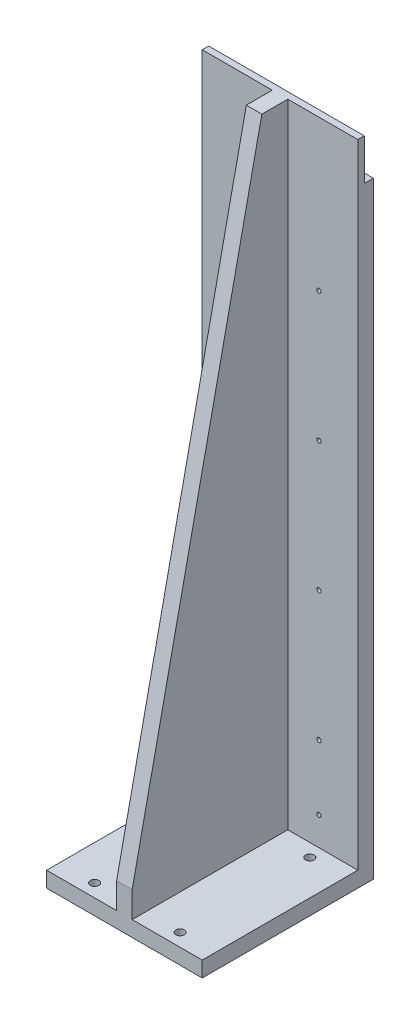
SolidWorks part; units mm, degrees
ref_plane "Front Plane" through (0, 0, 0) normal (0, 0, 1) x (1, 0, 0)
ref_plane "Top Plane" through (0, 0, 0) normal (0, 1, 0) x (1, 0, 0)
ref_plane "Right Plane" through (0, 0, 0) normal (1, 0, 0) x (0, 0, -1)
sketch "Sketch1" plane through (0, 0, 0) normal (0, 0, 1) x (1, 0, 0)
  line L1 (-60, 250) -> (60, 250)
  line L2 (-60, 250) -> (-60, -250)
  line L3 (-60, -250) -> (60, -250)
  line L4 (60, 250) -> (60, -250)
  line L5 (-60, 250) -> (60, -250) construction
  line L6 (-60, -250) -> (60, 250) construction
  point P0 (0, 0)
  dimension "D1" = 120
  dimension "D2" = 500
extrude "Boss-Extrude1" add sketch "Sketch1" along normal blind 12
sketch "Sketch2" plane through (0, 0, 12) normal (0, 0, 1) x (1, 0, 0)
  line L0 (60, -250) -> (60, 250) construction
  line L1 (-60, -250) -> (60, -250)
  line L2 (-60, -250) -> (-60, -238)
  line L3 (-60, -238) -> (60, -238)
  line L4 (60, -250) -> (60, -238)
  dimension "D1" = 12
extrude "Boss-Extrude2" add sketch "Sketch2" along normal blind 120
sketch "Sketch3" plane through (0, 0, 0) normal (1, 0, 0) x (0, 0, -1)
  line L0 (-12, 250) -> (-32, 250)
  line L1 (-12, -238) -> (-12, 250) construction
  line L2 (-32, 250) -> (-132, -218)
  line L3 (-132, -218) -> (-132, -238)
  line L4 (-132, -238) -> (-12, -238) construction
  line L5 (-132, -238) -> (-12, -238)
  line L6 (-12, -238) -> (-12, 250)
  line L8 (-12, 250) -> (0, 250) construction
  dimension "D1" = 20
  dimension "D2" = 20
extrude "Boss-Extrude3" add sketch "Sketch3" along normal mid plane 12
hole_wizard "M6 Clearance Hole1" positions "Sketch5" profile "Sketch4" hole size "M6" standard "GB"
sketch "Sketch5" plane through (0, -238, 0) normal (0, 1, 0) x (1, 0, 0)
  line L1 (33, -122) -> (33, -22) construction
  line L2 (60, -132) -> (60, -12) construction
  line L3 (6, -132) -> (6, -12) construction
  line L4 (60, -12) -> (6, -12) construction
  line L5 (6, -72) -> (33, -72) construction
  point P9 (33, -22)
  point P10 (33, -122)
  dimension "D1" = 10
sketch "Sketch4" plane through (33, -238, 122) normal (1, 0, 0) x (0, 0, 1)
  line L0 (0, 0) -> (0, 16.9828)
  line L1 (0, 16.9828) -> (3.3, 15)
  line L2 (3.3, 15) -> (3.3, 0)
  line L5 (3.3, 0) -> (0, 0)
  line L10 (0, 16.9828) -> (-3.3, 15) construction
  line L11 (0, -6.35) -> (0, 107.95) construction
  dimension "孔直径" = 6.6
  dimension "孔深度" = 15
  dimension "导头角度" = 118
hole_wizard "M6 Clearance Hole2" positions "Sketch7" profile "Sketch6" hole size "M6" standard "GB"
sketch "Sketch7" plane through (0, -238, 0) normal (0, 1, 0) x (1, 0, 0)
  line L1 (-33, -122) -> (-33, -22) construction
  line L2 (-60, -132) -> (-60, -12) construction
  line L3 (-6, -132) -> (-6, -12) construction
  line L4 (-6, -12) -> (-60, -12) construction
  line L5 (-6, -72) -> (-33, -72) construction
  point P9 (-33, -22)
  point P10 (-33, -122)
  dimension "D1" = 10
sketch "Sketch6" plane through (-33, -238, 122) normal (1, 0, 0) x (0, 0, 1)
  line L0 (0, 0) -> (0, 16.9828)
  line L1 (0, 16.9828) -> (3.3, 15)
  line L2 (3.3, 15) -> (3.3, 0)
  line L5 (3.3, 0) -> (0, 0)
  line L10 (0, 16.9828) -> (-3.3, 15) construction
  line L11 (0, -6.35) -> (0, 107.95) construction
  dimension "孔直径" = 6.6
  dimension "孔深度" = 15
  dimension "导头角度" = 118
hole_wizard "M4 Tapped Hole1" positions "Sketch9" profile "Sketch8" tap size "M4" standard "GB" end condition through all
sketch "Sketch9" plane through (0, 0, 0) normal (0, 0, -1) x (-1, 0, 0)
  point P1 (-30, 34)
  point P5 (-30, 134)
  point P9 (-30, -66)
  point P13 (-30, -166)
  point P17 (-30, -216)
  point P21 (30, -216)
  point P25 (30, -166)
  point P29 (30, -66)
  point P33 (30, 34)
  point P37 (30, 134)
  dimension "D1" = 30
  dimension "D2" = 30
  dimension "D3" = 50
  dimension "D4" = 100
  dimension "D5" = 66
  dimension "D6" = 34
  dimension "D7" = 100
sketch "Sketch8" plane through (30, 34, 0) normal (1, 0, 0) x (0, 1, 0)
  line L0 (0, 0) -> (0, 132)
  line L1 (0, 132) -> (1.65, 132)
  line L2 (1.65, 132) -> (1.65, 0)
  line L5 (1.65, 0) -> (0, 0)
  line L11 (0, -6.35) -> (0, 107.95) construction
  dimension "通孔螺纹孔钻头直径" = 3.3
  dimension "通孔螺纹孔钻头深度" = 132
cosmetic thread "Cosmetic Thread3" parameters "D2"=4
cosmetic thread "Cosmetic Thread4" parameters "D2"=4
cosmetic thread "Cosmetic Thread5" parameters "D2"=4
cosmetic thread "Cosmetic Thread6" parameters "D2"=4
cosmetic thread "Cosmetic Thread7" parameters "D2"=4
cosmetic thread "Cosmetic Thread8" parameters "D2"=4
cosmetic thread "Cosmetic Thread9" parameters "D2"=4
cosmetic thread "Cosmetic Thread10" parameters "D2"=4
cosmetic thread "Cosmetic Thread11" parameters "D2"=4
cosmetic thread "Cosmetic Thread12" parameters "D2"=4
sketch "Sketch10" plane through (60, 0, 0) normal (1, 0, 0) x (0, 0, -1)
  line L1 (0, 250) -> (-7, 250)
  line L2 (0, 250) -> (0, 218.2)
  line L3 (0, 218.2) -> (-7, 218.2)
  line L4 (-7, 250) -> (-7, 218.2)
  dimension "D1" = 7
  dimension "D2" = 31.8
extrude "Cut-Extrude1" cut sketch "Sketch10" against normal through all both and the other way through all
